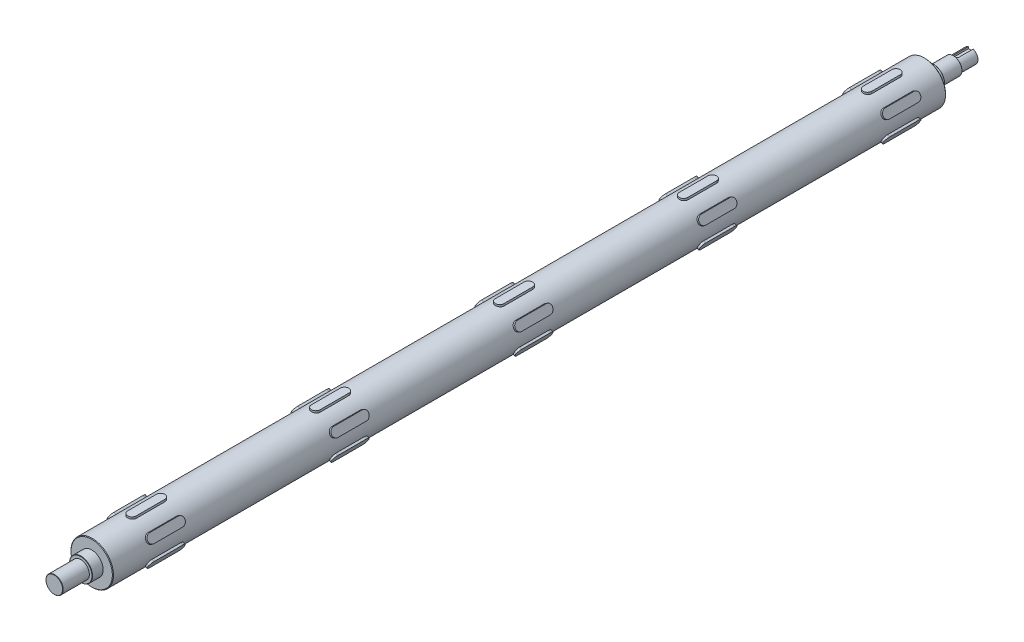
from build123d import *

# Parameters (mm, degrees)
SKETCH_1_R                       = 37
EXTRUDE_1_DEPTH                  = 1450
SKETCH_2_R                       = 20
EXTRUDE_2_DEPTH                  = 50
EXTRUDE_START                    = 45
SKETCH_3_R                       = 20
EXTRUDE_3_DEPTH                  = 45
EXTRUDE_4_DEPTH                  = 2.5
PATTERN_LINEAR_1_COUNT           = 5
PATTERN_LINEAR_1_PITCH           = 320
PATTERN_CIRCULAR_1_COUNT         = 6
PATTERN_CIRCULAR_1_COPY_1_DEPTH  = 2.5
PATTERN_CIRCULAR_1_COPY_2_DEPTH  = 2.5
PATTERN_CIRCULAR_1_COPY_3_DEPTH  = 2.5
PATTERN_CIRCULAR_1_COPY_4_DEPTH  = 2.5
PATTERN_CIRCULAR_1_COPY_5_DEPTH  = 2.5
PATTERN_CIRCULAR_1_COPY_6_DEPTH  = 2.5
PATTERN_CIRCULAR_1_COPY_7_DEPTH  = 2.5
PATTERN_CIRCULAR_1_COPY_8_DEPTH  = 2.5
PATTERN_CIRCULAR_1_COPY_9_DEPTH  = 2.5
PATTERN_CIRCULAR_1_COPY_10_DEPTH = 2.5
PATTERN_CIRCULAR_1_COPY_11_DEPTH = 2.5
PATTERN_CIRCULAR_1_COPY_12_DEPTH = 2.5
PATTERN_CIRCULAR_1_COPY_13_DEPTH = 2.5
PATTERN_CIRCULAR_1_COPY_14_DEPTH = 2.5
PATTERN_CIRCULAR_1_COPY_15_DEPTH = 2.5
PATTERN_CIRCULAR_1_COPY_16_DEPTH = 2.5
PATTERN_CIRCULAR_1_COPY_17_DEPTH = 2.5
PATTERN_CIRCULAR_1_COPY_18_DEPTH = 2.5
PATTERN_CIRCULAR_1_COPY_19_DEPTH = 2.5
PATTERN_CIRCULAR_1_COPY_20_DEPTH = 2.5
CHAMFER_1_SIZE                   = 1
SKETCH_6_OUTSIDE_W               = 388.576
SKETCH_6_OUTSIDE_H               = 391.794
SKETCH_6_OUTSIDE_R               = 15
CUT_EXTRUDE_1_DEPTH              = 35
SKETCH_7_OUTSIDE_W               = 388.576
SKETCH_7_OUTSIDE_H               = 391.794
SKETCH_7_OUTSIDE_R               = 15
CUT_EXTRUDE_2_DEPTH              = 26
SKETCH_8_R                       = 15
EXTRUDE_5_DEPTH                  = 20
CHAMFER_2_SIZE                   = 0.5
SKETCH_9_R                       = 12.5
EXTRUDE_6_DEPTH                  = 30
CUT_EXTRUDE_3_DEPTH              = 60
HOLE_WIZARD_M8_1_D               = 6.8
HOLE_WIZARD_M8_1_DEPTH           = 19.75
HOLE_WIZARD_M8_1_TIP             = 2.042926105


with BuildPart() as part:
    # 草图1 → 凸台-拉伸1 (new body)
    with BuildSketch(Plane.XY):
        Circle(SKETCH_1_R)
    extrude(amount=EXTRUDE_1_DEPTH)

    # 草图2 → 凸台-拉伸2 (add)
    with BuildSketch(Plane(origin=(0, 0, 0), x_dir=(-1, 0, 0), z_dir=(0, 0, -1))):
        with Locations(Location((0, 0, 0), (0, 0, 180))):
            Circle(SKETCH_2_R)
    extrude(amount=EXTRUDE_2_DEPTH)

    # 草图3 → 凸台-拉伸3 (add)
    with BuildSketch(Plane.XY.offset(1450).offset(EXTRUDE_START)):
        Circle(SKETCH_3_R)
    extrude(amount=-EXTRUDE_3_DEPTH)

    # 草图5 → 凸台-拉伸4 (add, symmetric)
    with BuildSketch(Plane(origin=(0, 37.5, 0), x_dir=(1, 0, 0), z_dir=(0, 1, 0))):
        with BuildLine():
            Line((-7.5, -100), (-7.5, -50))
            ThreePointArc((-7.5, -50), (0, -42.5), (7.5, -50))
            Line((7.5, -50), (7.5, -100))
            ThreePointArc((7.5, -100), (0, -107.5), (-7.5, -100))
        make_face()
    extrude_4 = extrude(amount=EXTRUDE_4_DEPTH, both=True)

    # 阵列(线性)1: 凸台-拉伸4 ×5
    with Locations(*[(0, 0, i * PATTERN_LINEAR_1_PITCH) for i in range(1, PATTERN_LINEAR_1_COUNT)]):
        add(extrude_4)

    # 阵列(圆周)1: 凸台-拉伸4 ×6 about axis
    pattern_circular_1_axis = Axis((0, 0, 0), (0, 0, 1))
    for i in range(1, PATTERN_CIRCULAR_1_COUNT):
        add(extrude_4.rotate(pattern_circular_1_axis, i * 360 / PATTERN_CIRCULAR_1_COUNT))

    # 阵列(圆周)1 copy 1 sketch → 阵列(圆周)1 copy 1 (add, symmetric)
    with BuildSketch(Plane(origin=(-32.475952642, 18.75, 320), x_dir=(0.5000000000000001, 0.8660254037844386, 0), z_dir=(-0.8660254037844386, 0.5000000000000001, 0))):
        with BuildLine():
            Line((-7.5, -100), (-7.5, -50))
            ThreePointArc((-7.5, -50), (0, -42.5), (7.5, -50))
            Line((7.5, -50), (7.5, -100))
            ThreePointArc((7.5, -100), (0, -107.5), (-7.5, -100))
        make_face()
    extrude(amount=PATTERN_CIRCULAR_1_COPY_1_DEPTH, both=True)

    # 阵列(圆周)1 copy 2 sketch → 阵列(圆周)1 copy 2 (add, symmetric)
    with BuildSketch(Plane(origin=(-32.475952642, -18.75, 320), x_dir=(-0.4999999999999998, 0.8660254037844387, 0), z_dir=(-0.8660254037844387, -0.4999999999999998, 0))):
        with BuildLine():
            Line((-7.5, -100), (-7.5, -50))
            ThreePointArc((-7.5, -50), (0, -42.5), (7.5, -50))
            Line((7.5, -50), (7.5, -100))
            ThreePointArc((7.5, -100), (0, -107.5), (-7.5, -100))
        make_face()
    extrude(amount=PATTERN_CIRCULAR_1_COPY_2_DEPTH, both=True)

    # 阵列(圆周)1 copy 3 sketch → 阵列(圆周)1 copy 3 (add, symmetric)
    with BuildSketch(Plane(origin=(0, -37.5, 320), x_dir=(-1, 0, 0), z_dir=(0, -1, 0))):
        with BuildLine():
            Line((-7.5, -100), (-7.5, -50))
            ThreePointArc((-7.5, -50), (0, -42.5), (7.5, -50))
            Line((7.5, -50), (7.5, -100))
            ThreePointArc((7.5, -100), (0, -107.5), (-7.5, -100))
        make_face()
    extrude(amount=PATTERN_CIRCULAR_1_COPY_3_DEPTH, both=True)

    # 阵列(圆周)1 copy 4 sketch → 阵列(圆周)1 copy 4 (add, symmetric)
    with BuildSketch(Plane(origin=(32.475952642, -18.75, 320), x_dir=(-0.5000000000000004, -0.8660254037844384, 0), z_dir=(0.8660254037844384, -0.5000000000000004, 0))):
        with BuildLine():
            Line((-7.5, -100), (-7.5, -50))
            ThreePointArc((-7.5, -50), (0, -42.5), (7.5, -50))
            Line((7.5, -50), (7.5, -100))
            ThreePointArc((7.5, -100), (0, -107.5), (-7.5, -100))
        make_face()
    extrude(amount=PATTERN_CIRCULAR_1_COPY_4_DEPTH, both=True)

    # 阵列(圆周)1 copy 5 sketch → 阵列(圆周)1 copy 5 (add, symmetric)
    with BuildSketch(Plane(origin=(32.475952642, 18.75, 320), x_dir=(0.5000000000000001, -0.8660254037844386, 0), z_dir=(0.8660254037844386, 0.5000000000000001, 0))):
        with BuildLine():
            Line((-7.5, -100), (-7.5, -50))
            ThreePointArc((-7.5, -50), (0, -42.5), (7.5, -50))
            Line((7.5, -50), (7.5, -100))
            ThreePointArc((7.5, -100), (0, -107.5), (-7.5, -100))
        make_face()
    extrude(amount=PATTERN_CIRCULAR_1_COPY_5_DEPTH, both=True)

    # 阵列(圆周)1 copy 6 sketch → 阵列(圆周)1 copy 6 (add, symmetric)
    with BuildSketch(Plane(origin=(-32.475952642, 18.75, 640), x_dir=(0.5000000000000001, 0.8660254037844386, 0), z_dir=(-0.8660254037844386, 0.5000000000000001, 0))):
        with BuildLine():
            Line((-7.5, -100), (-7.5, -50))
            ThreePointArc((-7.5, -50), (0, -42.5), (7.5, -50))
            Line((7.5, -50), (7.5, -100))
            ThreePointArc((7.5, -100), (0, -107.5), (-7.5, -100))
        make_face()
    extrude(amount=PATTERN_CIRCULAR_1_COPY_6_DEPTH, both=True)

    # 阵列(圆周)1 copy 7 sketch → 阵列(圆周)1 copy 7 (add, symmetric)
    with BuildSketch(Plane(origin=(-32.475952642, -18.75, 640), x_dir=(-0.4999999999999998, 0.8660254037844387, 0), z_dir=(-0.8660254037844387, -0.4999999999999998, 0))):
        with BuildLine():
            Line((-7.5, -100), (-7.5, -50))
            ThreePointArc((-7.5, -50), (0, -42.5), (7.5, -50))
            Line((7.5, -50), (7.5, -100))
            ThreePointArc((7.5, -100), (0, -107.5), (-7.5, -100))
        make_face()
    extrude(amount=PATTERN_CIRCULAR_1_COPY_7_DEPTH, both=True)

    # 阵列(圆周)1 copy 8 sketch → 阵列(圆周)1 copy 8 (add, symmetric)
    with BuildSketch(Plane(origin=(0, -37.5, 640), x_dir=(-1, 0, 0), z_dir=(0, -1, 0))):
        with BuildLine():
            Line((-7.5, -100), (-7.5, -50))
            ThreePointArc((-7.5, -50), (0, -42.5), (7.5, -50))
            Line((7.5, -50), (7.5, -100))
            ThreePointArc((7.5, -100), (0, -107.5), (-7.5, -100))
        make_face()
    extrude(amount=PATTERN_CIRCULAR_1_COPY_8_DEPTH, both=True)

    # 阵列(圆周)1 copy 9 sketch → 阵列(圆周)1 copy 9 (add, symmetric)
    with BuildSketch(Plane(origin=(32.475952642, -18.75, 640), x_dir=(-0.5000000000000004, -0.8660254037844384, 0), z_dir=(0.8660254037844384, -0.5000000000000004, 0))):
        with BuildLine():
            Line((-7.5, -100), (-7.5, -50))
            ThreePointArc((-7.5, -50), (0, -42.5), (7.5, -50))
            Line((7.5, -50), (7.5, -100))
            ThreePointArc((7.5, -100), (0, -107.5), (-7.5, -100))
        make_face()
    extrude(amount=PATTERN_CIRCULAR_1_COPY_9_DEPTH, both=True)

    # 阵列(圆周)1 copy 10 sketch → 阵列(圆周)1 copy 10 (add, symmetric)
    with BuildSketch(Plane(origin=(32.475952642, 18.75, 640), x_dir=(0.5000000000000001, -0.8660254037844386, 0), z_dir=(0.8660254037844386, 0.5000000000000001, 0))):
        with BuildLine():
            Line((-7.5, -100), (-7.5, -50))
            ThreePointArc((-7.5, -50), (0, -42.5), (7.5, -50))
            Line((7.5, -50), (7.5, -100))
            ThreePointArc((7.5, -100), (0, -107.5), (-7.5, -100))
        make_face()
    extrude(amount=PATTERN_CIRCULAR_1_COPY_10_DEPTH, both=True)

    # 阵列(圆周)1 copy 11 sketch → 阵列(圆周)1 copy 11 (add, symmetric)
    with BuildSketch(Plane(origin=(-32.475952642, 18.75, 960), x_dir=(0.5000000000000001, 0.8660254037844386, 0), z_dir=(-0.8660254037844386, 0.5000000000000001, 0))):
        with BuildLine():
            Line((-7.5, -100), (-7.5, -50))
            ThreePointArc((-7.5, -50), (0, -42.5), (7.5, -50))
            Line((7.5, -50), (7.5, -100))
            ThreePointArc((7.5, -100), (0, -107.5), (-7.5, -100))
        make_face()
    extrude(amount=PATTERN_CIRCULAR_1_COPY_11_DEPTH, both=True)

    # 阵列(圆周)1 copy 12 sketch → 阵列(圆周)1 copy 12 (add, symmetric)
    with BuildSketch(Plane(origin=(-32.475952642, -18.75, 960), x_dir=(-0.4999999999999998, 0.8660254037844387, 0), z_dir=(-0.8660254037844387, -0.4999999999999998, 0))):
        with BuildLine():
            Line((-7.5, -100), (-7.5, -50))
            ThreePointArc((-7.5, -50), (0, -42.5), (7.5, -50))
            Line((7.5, -50), (7.5, -100))
            ThreePointArc((7.5, -100), (0, -107.5), (-7.5, -100))
        make_face()
    extrude(amount=PATTERN_CIRCULAR_1_COPY_12_DEPTH, both=True)

    # 阵列(圆周)1 copy 13 sketch → 阵列(圆周)1 copy 13 (add, symmetric)
    with BuildSketch(Plane(origin=(0, -37.5, 960), x_dir=(-1, 0, 0), z_dir=(0, -1, 0))):
        with BuildLine():
            Line((-7.5, -100), (-7.5, -50))
            ThreePointArc((-7.5, -50), (0, -42.5), (7.5, -50))
            Line((7.5, -50), (7.5, -100))
            ThreePointArc((7.5, -100), (0, -107.5), (-7.5, -100))
        make_face()
    extrude(amount=PATTERN_CIRCULAR_1_COPY_13_DEPTH, both=True)

    # 阵列(圆周)1 copy 14 sketch → 阵列(圆周)1 copy 14 (add, symmetric)
    with BuildSketch(Plane(origin=(32.475952642, -18.75, 960), x_dir=(-0.5000000000000004, -0.8660254037844384, 0), z_dir=(0.8660254037844384, -0.5000000000000004, 0))):
        with BuildLine():
            Line((-7.5, -100), (-7.5, -50))
            ThreePointArc((-7.5, -50), (0, -42.5), (7.5, -50))
            Line((7.5, -50), (7.5, -100))
            ThreePointArc((7.5, -100), (0, -107.5), (-7.5, -100))
        make_face()
    extrude(amount=PATTERN_CIRCULAR_1_COPY_14_DEPTH, both=True)

    # 阵列(圆周)1 copy 15 sketch → 阵列(圆周)1 copy 15 (add, symmetric)
    with BuildSketch(Plane(origin=(32.475952642, 18.75, 960), x_dir=(0.5000000000000001, -0.8660254037844386, 0), z_dir=(0.8660254037844386, 0.5000000000000001, 0))):
        with BuildLine():
            Line((-7.5, -100), (-7.5, -50))
            ThreePointArc((-7.5, -50), (0, -42.5), (7.5, -50))
            Line((7.5, -50), (7.5, -100))
            ThreePointArc((7.5, -100), (0, -107.5), (-7.5, -100))
        make_face()
    extrude(amount=PATTERN_CIRCULAR_1_COPY_15_DEPTH, both=True)

    # 阵列(圆周)1 copy 16 sketch → 阵列(圆周)1 copy 16 (add, symmetric)
    with BuildSketch(Plane(origin=(-32.475952642, 18.75, 1280), x_dir=(0.5000000000000001, 0.8660254037844386, 0), z_dir=(-0.8660254037844386, 0.5000000000000001, 0))):
        with BuildLine():
            Line((-7.5, -100), (-7.5, -50))
            ThreePointArc((-7.5, -50), (0, -42.5), (7.5, -50))
            Line((7.5, -50), (7.5, -100))
            ThreePointArc((7.5, -100), (0, -107.5), (-7.5, -100))
        make_face()
    extrude(amount=PATTERN_CIRCULAR_1_COPY_16_DEPTH, both=True)

    # 阵列(圆周)1 copy 17 sketch → 阵列(圆周)1 copy 17 (add, symmetric)
    with BuildSketch(Plane(origin=(-32.475952642, -18.75, 1280), x_dir=(-0.4999999999999998, 0.8660254037844387, 0), z_dir=(-0.8660254037844387, -0.4999999999999998, 0))):
        with BuildLine():
            Line((-7.5, -100), (-7.5, -50))
            ThreePointArc((-7.5, -50), (0, -42.5), (7.5, -50))
            Line((7.5, -50), (7.5, -100))
            ThreePointArc((7.5, -100), (0, -107.5), (-7.5, -100))
        make_face()
    extrude(amount=PATTERN_CIRCULAR_1_COPY_17_DEPTH, both=True)

    # 阵列(圆周)1 copy 18 sketch → 阵列(圆周)1 copy 18 (add, symmetric)
    with BuildSketch(Plane(origin=(0, -37.5, 1280), x_dir=(-1, 0, 0), z_dir=(0, -1, 0))):
        with BuildLine():
            Line((-7.5, -100), (-7.5, -50))
            ThreePointArc((-7.5, -50), (0, -42.5), (7.5, -50))
            Line((7.5, -50), (7.5, -100))
            ThreePointArc((7.5, -100), (0, -107.5), (-7.5, -100))
        make_face()
    extrude(amount=PATTERN_CIRCULAR_1_COPY_18_DEPTH, both=True)

    # 阵列(圆周)1 copy 19 sketch → 阵列(圆周)1 copy 19 (add, symmetric)
    with BuildSketch(Plane(origin=(32.475952642, -18.75, 1280), x_dir=(-0.5000000000000004, -0.8660254037844384, 0), z_dir=(0.8660254037844384, -0.5000000000000004, 0))):
        with BuildLine():
            Line((-7.5, -100), (-7.5, -50))
            ThreePointArc((-7.5, -50), (0, -42.5), (7.5, -50))
            Line((7.5, -50), (7.5, -100))
            ThreePointArc((7.5, -100), (0, -107.5), (-7.5, -100))
        make_face()
    extrude(amount=PATTERN_CIRCULAR_1_COPY_19_DEPTH, both=True)

    # 阵列(圆周)1 copy 20 sketch → 阵列(圆周)1 copy 20 (add, symmetric)
    with BuildSketch(Plane(origin=(32.475952642, 18.75, 1280), x_dir=(0.5000000000000001, -0.8660254037844386, 0), z_dir=(0.8660254037844386, 0.5000000000000001, 0))):
        with BuildLine():
            Line((-7.5, -100), (-7.5, -50))
            ThreePointArc((-7.5, -50), (0, -42.5), (7.5, -50))
            Line((7.5, -50), (7.5, -100))
            ThreePointArc((7.5, -100), (0, -107.5), (-7.5, -100))
        make_face()
    extrude(amount=PATTERN_CIRCULAR_1_COPY_20_DEPTH, both=True)

    # 倒角1
    chamfer_1_edges = [part.edges().sort_by_distance(p)[0] for p in [
        (-37, 0, 0),
        (-37, 0, 1450),
    ]]
    chamfer(chamfer_1_edges, length=CHAMFER_1_SIZE)

    # 草图6 outside → 切除-拉伸1 (cut)
    with BuildSketch(Plane(origin=(0, 0, -50), x_dir=(-1, 0, 0), z_dir=(0, 0, -1))):
        Rectangle(SKETCH_6_OUTSIDE_W, SKETCH_6_OUTSIDE_H)
        Circle(SKETCH_6_OUTSIDE_R, mode=Mode.SUBTRACT)
    extrude(amount=-CUT_EXTRUDE_1_DEPTH, mode=Mode.SUBTRACT)

    # 草图7 outside → 切除-拉伸2 (cut)
    with BuildSketch(Plane.XY.offset(1495)):
        Rectangle(SKETCH_7_OUTSIDE_W, SKETCH_7_OUTSIDE_H)
        with Locations(Location((0, 0, 0), (0, 0, 180))):
            Circle(SKETCH_7_OUTSIDE_R, mode=Mode.SUBTRACT)
    extrude(amount=-CUT_EXTRUDE_2_DEPTH, mode=Mode.SUBTRACT)

    # 草图8 → 凸台-拉伸5 (add)
    with BuildSketch(Plane.XY.offset(1495)):
        with Locations(Location((0, 0, 0), (0, 0, 180))):
            Circle(SKETCH_8_R)
    extrude(amount=EXTRUDE_5_DEPTH)

    # 倒角2
    chamfer_2_edges = [part.edges().sort_by_distance(p)[0] for p in [
        (-20, 0, -15),
        (15, 0, -50),
        (-20, 0, 1469),
        (15, 0, 1515),
    ]]
    chamfer(chamfer_2_edges, length=CHAMFER_2_SIZE)

    # 草图9 → 凸台-拉伸6 (add)
    with BuildSketch(Plane(origin=(0, 0, -50), x_dir=(-1, 0, 0), z_dir=(0, 0, -1))):
        Circle(SKETCH_9_R)
    extrude(amount=EXTRUDE_6_DEPTH)

    # 草图10 → 切除-拉伸3 (cut)
    with BuildSketch(Plane(origin=(0, 8.5, 0), x_dir=(1, 0, 0), z_dir=(0, 1, 0))):
        with BuildLine():
            Line((4, 80), (4, 55))
            ThreePointArc((4, 55), (0, 51), (-4, 55))
            Line((-4, 55), (-4, 80))
            ThreePointArc((-4, 80), (0, 84), (4, 80))
        make_face()
    extrude(amount=CUT_EXTRUDE_3_DEPTH, mode=Mode.SUBTRACT)

    # M8 螺纹孔1
    with Locations(Plane(origin=(0, 0, -80), x_dir=(-1, 0, 0), z_dir=(0, 0, -1))):
        with Locations((0, 0)):
            Hole(HOLE_WIZARD_M8_1_D / 2, depth=HOLE_WIZARD_M8_1_DEPTH)
            with Locations((0, 0, -(HOLE_WIZARD_M8_1_DEPTH + HOLE_WIZARD_M8_1_TIP / 2))):  # 118° drill point
                Cone(0, HOLE_WIZARD_M8_1_D / 2, HOLE_WIZARD_M8_1_TIP, mode=Mode.SUBTRACT)


solid = part.part
